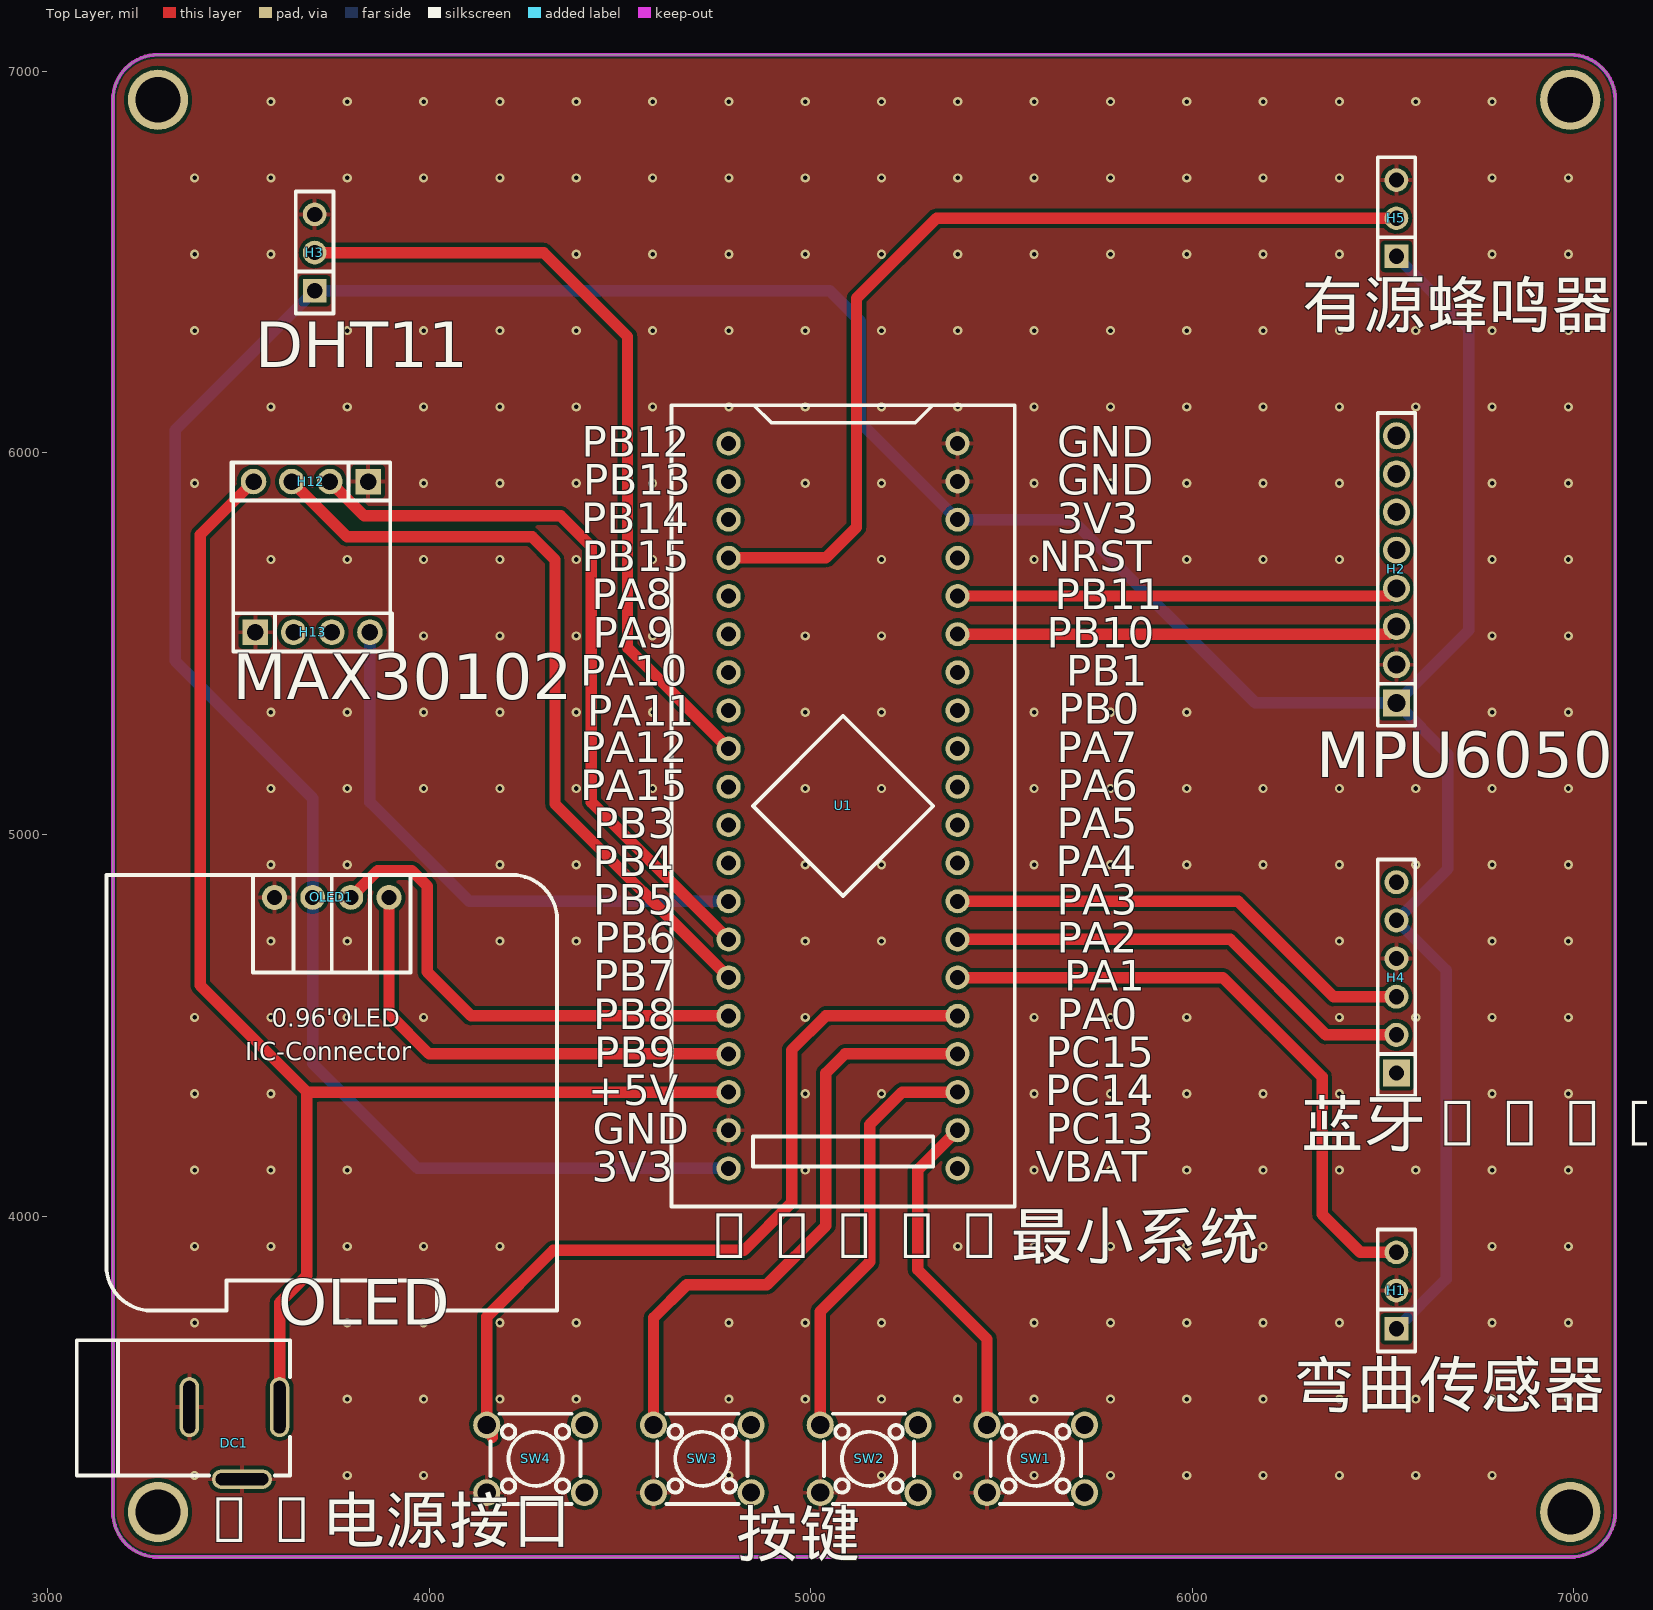
[diagram p0: Top Layer view]
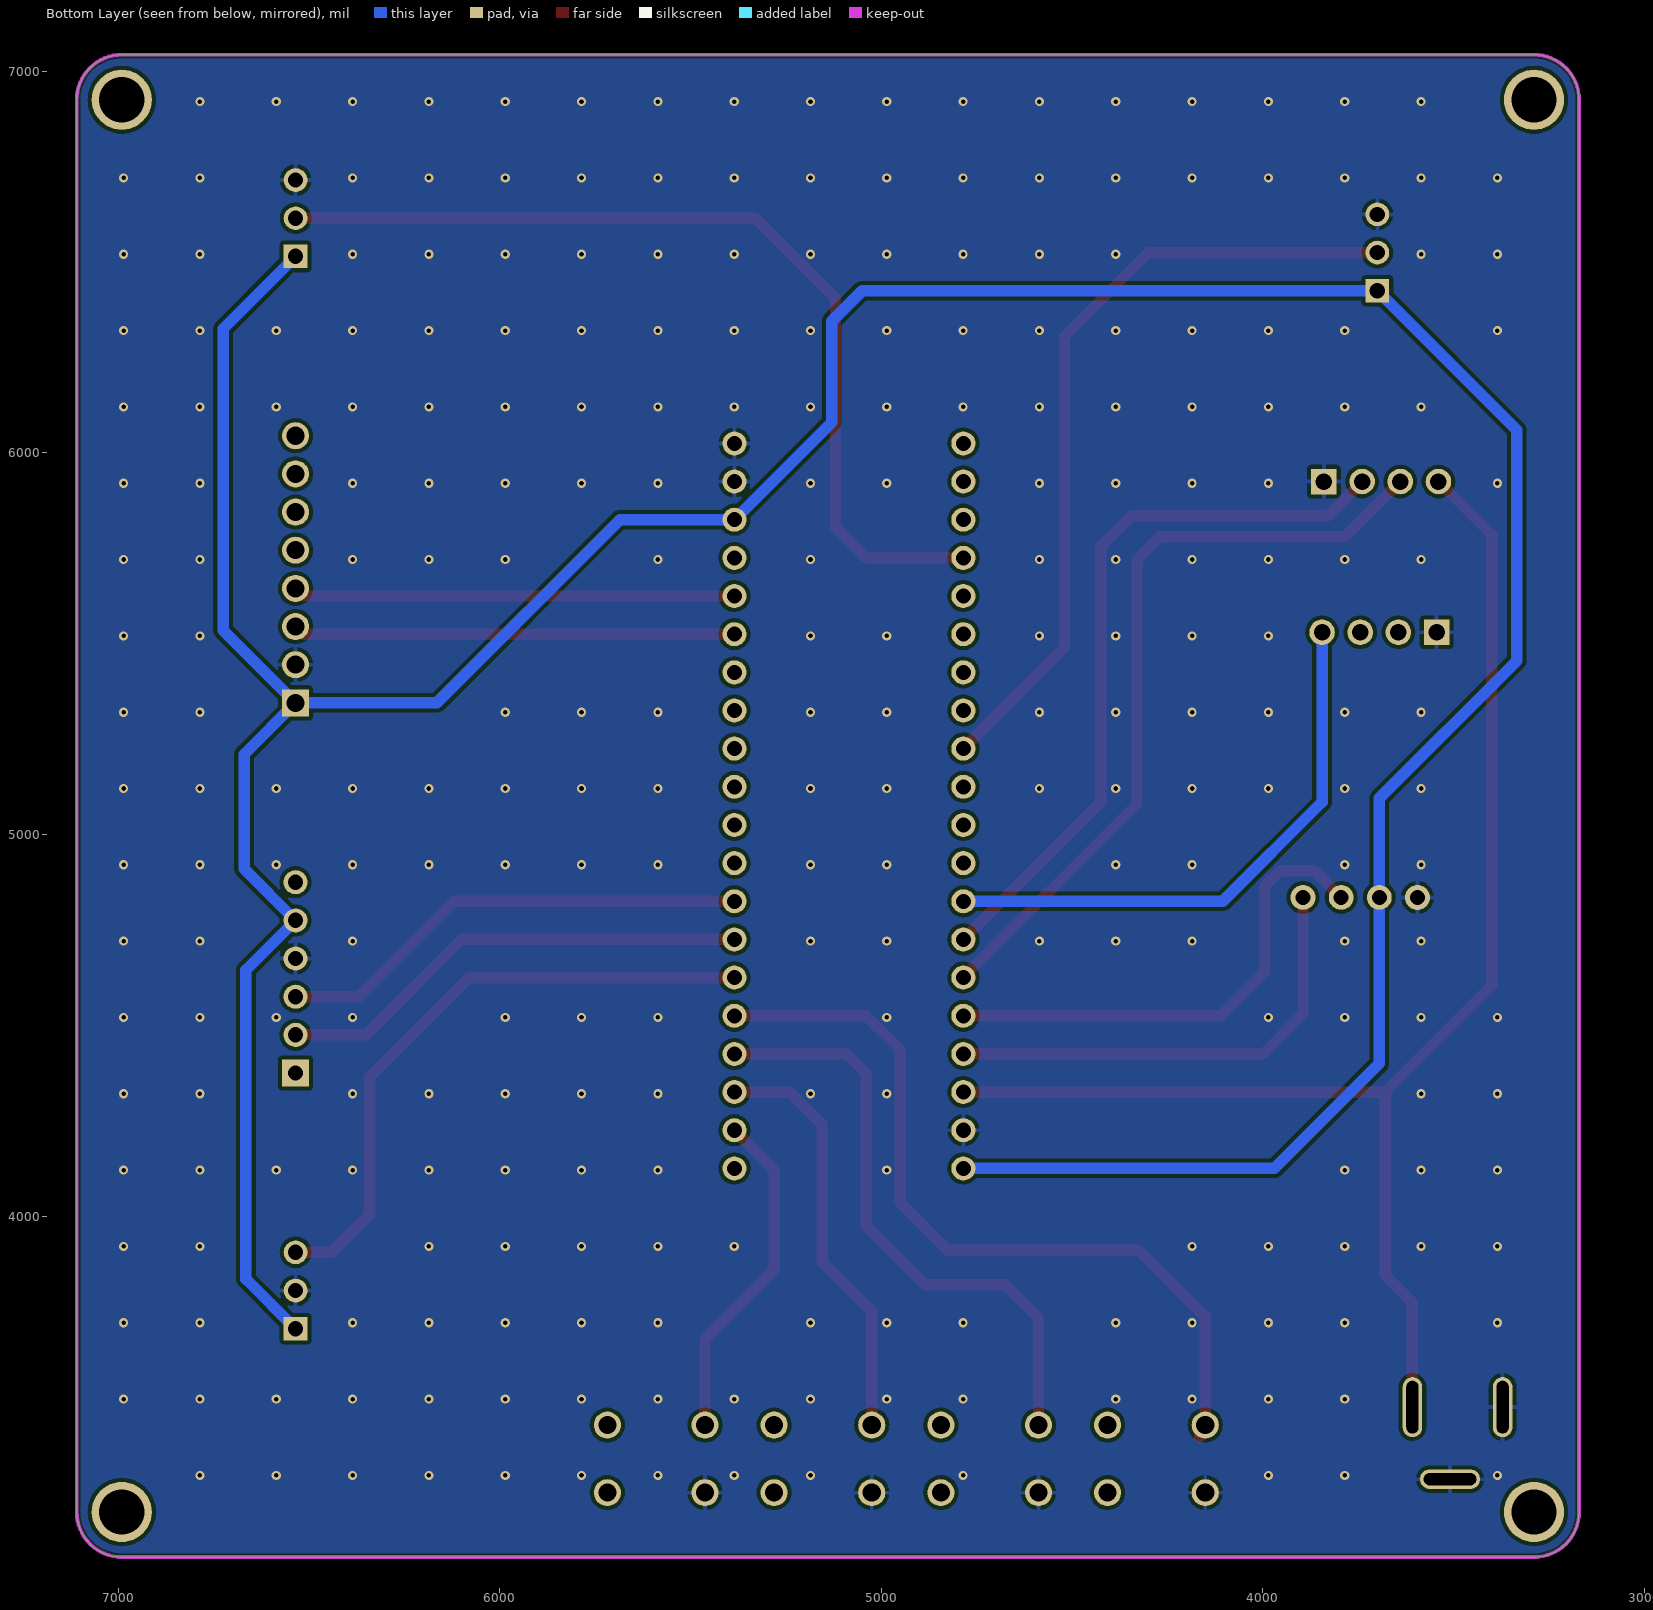
[diagram p1: Bottom Layer view, seen from below]
# Altium PCB MISC51890.pcbdoc
Units mil, origin at the board's own origin, x right, y up, seen from the top; angles counter-clockwise.
Board outline 3937.01 x 3937.01 mil, 2 copper layers (Top Layer, Bottom Layer), stack 62.206 mil thick; 14 components, 37 nets, 98 pads, 265 vias.

## Layer stack, top to bottom
Top Solder Mask Layer: solder mask 0.394, Dk 3.3
Top Layer: signal copper 1.379
Dielectric1: surface 59.449, FR4, Dk 4.5
Bottom Layer: signal copper 1.378
Bottom Solder Mask Layer: solder mask 0.394, Dk 3.3

## Board outline
6990.39,3106.5 ccw(c6990.39,3224.61) 7108.5,3224.61 7108.5,6925.39 ccw(c6990.39,6925.39) 6990.39,7043.5 3289.61,7043.5 ccw(c3289.61,6925.39) 3171.5,6925.39 3171.5,3224.61 ccw(c3289.61,3224.61) 3289.61,3106.5

## Design rules (kind name [scope] priority, off if disabled: settings)
BoardOutlineClearance copperThickness2oz_1 [All] p2 off: genericclearance=7.99 ignorepadtopadclearanceinfootprint=FALSE except(0: Arc-SplitContinuation Track-SplitContinuation SMDPad-SplitContinuation THPad-SplitContinuation Via-SplitContinuation Fill-SplitContinuation Region-SplitContinuation Poly-SplitContinuation Text-SplitContinuation Hole-SplitContinuation; 5.98: Arc-CutoutEdge Track-CutoutEdge SMDPad-CutoutEdge THPad-CutoutEdge Via-CutoutEdge Text-CutoutEdge; 6.89: Hole-OutlineEdge Hole-CutoutEdge; 10: Poly-OutlineEdge Poly-CutoutEdge; 11.81: Arc-OutlineEdge Track-OutlineEdge SMDPad-OutlineEdge THPad-OutlineEdge Via-OutlineEdge Fill-OutlineEdge Region-OutlineEdge Text-OutlineEdge Fill-CutoutEdge Region-CutoutEdge)
BoardOutlineClearance Plane_innerPlane_1 [All] p4 off: genericclearance=4.02 ignorepadtopadclearanceinfootprint=FALSE except(0: Arc-SplitContinuation Track-SplitContinuation SMDPad-SplitContinuation THPad-SplitContinuation Via-SplitContinuation Fill-SplitContinuation Region-SplitContinuation Poly-SplitContinuation Text-SplitContinuation Hole-SplitContinuation; 5.98: Arc-CutoutEdge Track-CutoutEdge SMDPad-CutoutEdge THPad-CutoutEdge Via-CutoutEdge Text-CutoutEdge; 6.89: Hole-OutlineEdge Hole-CutoutEdge; 10: Poly-OutlineEdge Poly-CutoutEdge; 11.81: Arc-OutlineEdge Track-OutlineEdge SMDPad-OutlineEdge THPad-OutlineEdge Via-OutlineEdge Fill-OutlineEdge Region-OutlineEdge Text-OutlineEdge Fill-CutoutEdge Region-CutoutEdge)
BoardOutlineClearance Copper_copperRegion_1 [All] p6 off: genericclearance=4.02 ignorepadtopadclearanceinfootprint=FALSE except(0: Arc-SplitContinuation Track-SplitContinuation SMDPad-SplitContinuation THPad-SplitContinuation Via-SplitContinuation Fill-SplitContinuation Region-SplitContinuation Poly-SplitContinuation Text-SplitContinuation Hole-SplitContinuation; 5.98: Arc-CutoutEdge Track-CutoutEdge SMDPad-CutoutEdge THPad-CutoutEdge Via-CutoutEdge Text-CutoutEdge; 6.89: Hole-OutlineEdge Hole-CutoutEdge; 10: Poly-OutlineEdge Poly-CutoutEdge; 11.81: Arc-OutlineEdge Track-OutlineEdge SMDPad-OutlineEdge THPad-OutlineEdge Via-OutlineEdge Fill-OutlineEdge Region-OutlineEdge Text-OutlineEdge Fill-CutoutEdge Region-CutoutEdge)
BoardOutlineClearance copperThickness1oz_1 [All] p8: genericclearance=4.02 ignorepadtopadclearanceinfootprint=FALSE except(0: Arc-SplitContinuation Track-SplitContinuation SMDPad-SplitContinuation THPad-SplitContinuation Via-SplitContinuation Fill-SplitContinuation Region-SplitContinuation Poly-SplitContinuation Text-SplitContinuation Hole-SplitContinuation; 5.98: Arc-CutoutEdge Track-CutoutEdge SMDPad-CutoutEdge THPad-CutoutEdge Via-CutoutEdge Text-CutoutEdge; 6.89: Hole-OutlineEdge Hole-CutoutEdge; 10: Poly-OutlineEdge Poly-CutoutEdge; 11.81: Arc-OutlineEdge Track-OutlineEdge SMDPad-OutlineEdge THPad-OutlineEdge Via-OutlineEdge Fill-OutlineEdge Region-OutlineEdge Text-OutlineEdge Fill-CutoutEdge Region-CutoutEdge)
Clearance copperThickness2oz [All] p1 off: gap=7.99 ignorepadtopadclearanceinfootprint=FALSE except(5.98: SMDPad-Track SMDPad-SMDPad THPad-Track SMDPad-THPad THPad-THPad Track-Via SMDPad-Via THPad-Via Via-Via Fill-SMDPad Region-SMDPad Fill-THPad Region-THPad Fill-Via Region-Via Fill-Fill Fill-Region Region-Region Arc-Track Arc-SMDPad Arc-THPad Arc-Via Fill-Arc Region-Arc Arc-Arc Text-Track SMDPad-Text Text-THPad Text-Via Fill-Text Region-Text Arc-Text Text-Text; 6.89: Hole-Track Hole-SMDPad Hole-THPad Hole-Via Fill-Hole Region-Hole Hole-Arc Hole-Text; 10: Poly-Track Poly-SMDPad Poly-THPad Poly-Via Poly-Fill Poly-Region Poly-Poly Poly-Arc Poly-Text Poly-Hole; 11.81: Fill-Track Region-Track)
Clearance Plane_innerPlane [All] p3 off: gap=4.02 ignorepadtopadclearanceinfootprint=FALSE except(5.98: SMDPad-Track SMDPad-SMDPad THPad-Track SMDPad-THPad THPad-THPad Track-Via SMDPad-Via THPad-Via Via-Via Fill-SMDPad Region-SMDPad Fill-THPad Region-THPad Fill-Via Region-Via Fill-Fill Fill-Region Region-Region Arc-Track Arc-SMDPad Arc-THPad Arc-Via Fill-Arc Region-Arc Arc-Arc Text-Track SMDPad-Text Text-THPad Text-Via Fill-Text Region-Text Arc-Text Text-Text; 6.89: Hole-Track Hole-SMDPad Hole-THPad Hole-Via Fill-Hole Region-Hole Hole-Arc Hole-Text; 10: Poly-Track Poly-SMDPad Poly-THPad Poly-Via Poly-Fill Poly-Region Poly-Poly Poly-Arc Poly-Text Poly-Hole; 11.81: Fill-Track Region-Track)
Clearance Copper_copperRegion [All] p5 off: gap=4.02 ignorepadtopadclearanceinfootprint=FALSE except(5.98: SMDPad-Track SMDPad-SMDPad THPad-Track SMDPad-THPad THPad-THPad Track-Via SMDPad-Via THPad-Via Via-Via Fill-SMDPad Region-SMDPad Fill-THPad Region-THPad Fill-Via Region-Via Fill-Fill Fill-Region Region-Region Arc-Track Arc-SMDPad Arc-THPad Arc-Via Fill-Arc Region-Arc Arc-Arc Text-Track SMDPad-Text Text-THPad Text-Via Fill-Text Region-Text Arc-Text Text-Text; 6.89: Hole-Track Hole-SMDPad Hole-THPad Hole-Via Fill-Hole Region-Hole Hole-Arc Hole-Text; 10: Poly-Track Poly-SMDPad Poly-THPad Poly-Via Poly-Fill Poly-Region Poly-Poly Poly-Arc Poly-Text Poly-Hole; 11.81: Fill-Track Region-Track)
Clearance copperThickness1oz [All] p7: gap=4.02 ignorepadtopadclearanceinfootprint=FALSE except(5.98: SMDPad-Track SMDPad-SMDPad THPad-Track SMDPad-THPad THPad-THPad Track-Via SMDPad-Via THPad-Via Via-Via Fill-SMDPad Region-SMDPad Fill-THPad Region-THPad Fill-Via Region-Via Fill-Fill Fill-Region Region-Region Arc-Track Arc-SMDPad Arc-THPad Arc-Via Fill-Arc Region-Arc Arc-Arc Text-Track SMDPad-Text Text-THPad Text-Via Fill-Text Region-Text Arc-Text Text-Text; 6.89: Hole-Track Hole-SMDPad Hole-THPad Hole-Via Fill-Hole Region-Hole Hole-Arc Hole-Text; 10: Poly-Track Poly-SMDPad Poly-THPad Poly-Via Poly-Fill Poly-Region Poly-Poly Poly-Arc Poly-Text Poly-Hole; 11.81: Fill-Track Region-Track)
DiffPairsRouting differentialPair [All] p1: maxlimit=6 minlimit=6 mostfreqgap=6 toplayer_minwidth=5 toplayer_prefwidth=10 toplayer_maxwidth=100 toplayer_mingap=6 toplayer_prefgap=6 toplayer_maxgap=6 bottomlayer_minwidth=5 bottomlayer_prefwidth=10 bottomlayer_maxwidth=100 bottomlayer_mingap=6 bottomlayer_prefgap=6 bottomlayer_maxgap=6 maxuncoupledlength=10
HoleToHoleClearance otherClearance [All] p1: gap=11.81 allowstackedmicrovias=TRUE
Length netLength [All] p1: minlimit=0 maxlimit=0
PasteMaskExpansion pasteMaskExpansion [All] p1: expansion=0
PlaneConnect innerPlane [All] p1: planeconnectstyle=Relief reliefexpansion=20 reliefentries=4 reliefconductorwidth=10 reliefairgap=10
PolygonConnect copperRegion [All] p1: connectstyle=Relief reliefconductorwidth=10 reliefentries=4 polygonreliefangle="90 Angle" airgapwidth=10 via.connectstyle=Relief via.reliefconductorwidth=10 via.reliefentries=4 via.polygonreliefangle="90 Angle" via.airgapwidth=10
RoutingVias viaSize [All] p1: holewidth=12.01 width=24.02 viastyle="Through Hole" minholewidth=11.81 minwidth=19.68 maxholewidth=248.03 maxwidth=393.7
SolderMaskExpansion solderMaskExpansion [IsVia] p1: expansion=-1000 istentingtop=TRUE
SolderMaskExpansion solderMaskExpansion [All] p2: expansion=2.01 istentingtop=FALSE
Width copperThickness2oz_2 [All] p1 off: maxlimit=100 minlimit=8 preferedwidth=10
Width copperThickness1oz_2 [All] p2: maxlimit=100 minlimit=5 preferedwidth=30

## Components (designator, comment, footprint, x,y, rotation, side; value= is the part's Value field where it differs from the comment)
DC1 "" DC-2.0 3485,3510 r180 top
H1 "" HDR-TH_3P-P2.54-V-F 6535,3805 r90 top
H2 "" HDR-TH_8P-P2.54-V-F-1 6535,5695 r90 top
H3 "" HDR-TH_3P-P2.54-V-F 3700,6525 r90 top
H4 "" HDR-TH_6P-P2.54-V-F 6535,4625 r90 top
H5 "" HDR-TH_3P-P2.54-V-F 6535,6615 r90 top
H12 "" HDR-TH_4P-P2.54-V-F 3690,5925 r180 top
H13 "" HDR-TH_4P-P2.54-V-F 3695,5530 r0 top
OLED1 "" 0.96OLED_4P 3745,4835 r0 top
SW1 "" SW-TH_4P-L6.0-W6.0-P4.50-LS6.5 5590,3363.89 r0 top
SW2 "" SW-TH_4P-L6.0-W6.0-P4.50-LS6.5 5153.02,3363.89 r0 top
SW3 "" SW-TH_4P-L6.0-W6.0-P4.50-LS6.5 4716.04,3363.89 r0 top
SW4 "" SW-TH_4P-L6.0-W6.0-P4.50-LS6.5 4279.06,3363.89 r0 top
U1 "STM32F103C8T6-Card" CONN-TH_L53.3-W22.9_STM32F103C8T6-CARD 5085,5075 r270 top

## Footprints (in the part's own frame and the unit in brackets; to place one, negate y for a bottom-side part, rotate by r counter-clockwise, add the part's x,y. Pads: shape width x height; smd on the part's side, far side on the other; paste and mask are expansions set on the pad)
0.96OLED_4P [mm]
  round 1.65 hole 1 copper offset 0,0: 1(-3.81,-0.001) 2(-1.27,0.002) 3(1.27,0.002) 4(3.81,0.002)
  silkscreen extent -15,-27.5 15,1.5
CONN-TH_L53.3-W22.9_STM32F103C8T6-CARD [mm]
  round 1.6 hole 1: 1(-24.13,-7.62) 2(-21.59,-7.62) 3(-19.05,-7.62) 4(-16.51,-7.62) 5(-13.97,-7.62) 6(-11.43,-7.62) 7(-8.89,-7.62) 8(-6.35,-7.62) 9(-3.81,-7.62) 10(-1.27,-7.62) 11(1.27,-7.62) 12(3.81,-7.62) 13(6.35,-7.62) 14(8.89,-7.62) 15(11.43,-7.62) 16(13.97,-7.62) 17(16.51,-7.62) 18(19.05,-7.62) 19(21.59,-7.62) 20(24.13,-7.62) 21(24.13,7.62) 22(21.59,7.62) 23(19.05,7.62) 24(16.51,7.62) 25(13.97,7.62) 26(11.43,7.62) 27(8.89,7.62) 28(6.35,7.62) 29(3.81,7.62) 30(1.27,7.62) 31(-1.27,7.62) 32(-3.81,7.62) 33(-6.35,7.62) 34(-8.89,7.62) 35(-11.43,7.62) 36(-13.97,7.62) 37(-16.51,7.62) 38(-19.05,7.62) 39(-21.59,7.62) 40(-24.13,7.62)
  silkscreen extent -26.67,-11.43 26.67,11.43
DC-2.0 [mil]
  oval 157.5x51.2 hole 31.5 slot 137.8 at 0 deg paste+0 mask+2: 2(-24.7,199.5)
  oval 51.2x157.5 hole 31.5 slot 137.8 at 90 deg paste+0 mask+2: 3(113.1,10.5) 4(-123.1,10.5)
  silkscreen extent -151,-165 408,190
HDR-TH_3P-P2.54-V-F [mil]
  rect 62x62 hole 40.16: 1(-100,0)
  round 62 hole 40.16: 2(0,0) 3(100,0)
  silkscreen extent -160,-49 160,49
HDR-TH_4P-P2.54-V-F [mm]
  rect 1.7x1.7 hole 1.1: 1(-3.81,0)
  round 1.7 hole 1.1: 2(-1.27,0) 3(1.27,0) 4(3.81,0)
  silkscreen extent -5.29,-1.27 5.29,1.27
HDR-TH_6P-P2.54-V-F [mm]
  rect 1.8x1.8 hole 1.02: 1(-6.35,0)
  round 1.6 hole 1.02: 2(-3.81,0) 3(-1.27,0) 4(1.27,0) 5(3.81,0) 6(6.35,0)
  silkscreen extent -7.87,-1.25 7.87,1.25
HDR-TH_8P-P2.54-V-F-1 [mm]
  rect 1.8x1.8 hole 1.2: 1(-8.89,0)
  round 1.8 hole 1.2: 2(-6.35,0) 3(-3.81,0) 4(-1.27,0) 5(1.27,0) 6(3.81,0) 7(6.35,0) 8(8.89,0)
  silkscreen extent -10.41,-1.25 10.41,1.25
SW-TH_4P-L6.0-W6.0-P4.50-LS6.5 [mm]
  round 1.8 hole 1.2: 1(-3.25,2.25) 2(3.25,2.25) 3(-3.25,-2.25) 4(3.25,-2.25)
  silkscreen extent -3,-3 3,3

## Free pads (board coordinates)
  round 157.48 hole 118.11: 1(3289.61,6925.39) 1(3289.61,3224.61) 1(6990.39,6925.39) 1(6990.39,3224.61)

## Via types
v1: diameter 24.02, hole 12, Top Layer to Bottom Layer, 265 vias

## Nets (pads, with @x,y where several pads share a name; then routed paths per layer and width w, separated by ;. In a path a pad name is that pad's centre, name@x,y a point inside that pad or via, vN(x,y) a via of type N, cw(c..) or ccw(c..) an arc to the next point about the centre after c; other vN are vias at no path point)
+5V: DC1.4 H12.4 U1.18 | length 3734.3
  Top Layer w30: H12.4 3400,5785 3400,4605 3680,4325 ; DC1.4 3608.1,3773.1 3680,3845 3680,4325 ; U1.18 3680,4325
GND: DC1.2 DC1.3 H1.2 H2.2 H3.3 H4.4 H5.3 H12.1 H13.1 OLED1.1 SW1.3 SW2.3 SW3.3 SW4.3 U1.19 U1.39 U1.40
  other v1: 3385.6,3320.6 3785.6,3320.6 3985.6,3320.6 4785.6,3320.6 5185.6,3320.6 5385.6,3320.6 5585.6,3320.6 5785.6,3320.6 5985.6,3320.6 6185.6,3320.6 6385.6,3320.6 6585.6,3320.6 6785.6,3320.6 3785.6,3520.6 3985.6,3520.6 4185.6,3520.6 4385.6,3520.6 4785.6,3520.6 4985.6,3520.6 5185.6,3520.6 5385.6,3520.6 5585.6,3520.6 5785.6,3520.6 5985.6,3520.6 6185.6,3520.6 6385.6,3520.6 6585.6,3520.6 6785.6,3520.6 6985.6,3520.6 3385.6,3720.6 3785.6,3720.6 3985.6,3720.6 4185.6,3720.6 4385.6,3720.6 4785.6,3720.6 4985.6,3720.6 5185.6,3720.6 5585.6,3720.6 5785.6,3720.6 5985.6,3720.6 6185.6,3720.6 6385.6,3720.6 6785.6,3720.6 6985.6,3720.6 3385.6,3920.6 3585.6,3920.6 3785.6,3920.6 3985.6,3920.6 4185.6,3920.6 5385.6,3920.6 5585.6,3920.6 5785.6,3920.6 5985.6,3920.6 6185.6,3920.6 6785.6,3920.6 6985.6,3920.6 3385.6,4120.6 3585.6,4120.6 3785.6,4120.6 4985.6,4120.6 5585.6,4120.6 5785.6,4120.6 5985.6,4120.6 6185.6,4120.6 6385.6,4120.6 6585.6,4120.6 6785.6,4120.6 6985.6,4120.6 3385.6,4320.6 3585.6,4320.6 4985.6,4320.6 5185.6,4320.6 5585.6,4320.6 5785.6,4320.6 5985.6,4320.6 6185.6,4320.6 6385.6,4320.6 6785.6,4320.6 6985.6,4320.6 3385.6,4520.6 3585.6,4520.6 3785.6,4520.6 3985.6,4520.6 4985.6,4520.6 5585.6,4520.6 5785.6,4520.6 5985.6,4520.6 6385.6,4520.6 6585.6,4520.6 6785.6,4520.6 6985.6,4520.6 3585.6,4720.6 3785.6,4720.6 4185.6,4720.6 4385.6,4720.6 4585.6,4720.6 4985.6,4720.6 5185.6,4720.6 6385.6,4720.6 6785.6,4720.6 6985.6,4720.6 3585.6,4920.6 3785.6,4920.6 4185.6,4920.6 4385.6,4920.6 4985.6,4920.6 5185.6,4920.6 5585.6,4920.6 5785.6,4920.6 5985.6,4920.6 6185.6,4920.6 6385.6,4920.6 6585.6,4920.6 6785.6,4920.6 6985.6,4920.6 3585.6,5120.6 3785.6,5120.6 3985.6,5120.6 4185.6,5120.6 4385.6,5120.6 4585.6,5120.6 4985.6,5120.6 5185.6,5120.6 5585.6,5120.6 5785.6,5120.6 5985.6,5120.6 6185.6,5120.6 6385.6,5120.6 6585.6,5120.6 6785.6,5120.6 6985.6,5120.6 3585.6,5320.6 3785.6,5320.6 3985.6,5320.6 4185.6,5320.6 4385.6,5320.6 4585.6,5320.6 4985.6,5320.6 5185.6,5320.6 5585.6,5320.6 5785.6,5320.6 5985.6,5320.6 6785.6,5320.6 6985.6,5320.6 3985.6,5520.6 4185.6,5520.6 4385.6,5520.6 4585.6,5520.6 4985.6,5520.6 5185.6,5520.6 6785.6,5520.6 6985.6,5520.6 3585.6,5720.6 3785.6,5720.6 3985.6,5720.6 4185.6,5720.6 4385.6,5720.6 4585.6,5720.6 5185.6,5720.6 5585.6,5720.6 5985.6,5720.6 6185.6,5720.6 6385.6,5720.6 6785.6,5720.6 6985.6,5720.6 3385.6,5920.6 3985.6,5920.6 4185.6,5920.6 4385.6,5920.6 4585.6,5920.6 4985.6,5920.6 5185.6,5920.6 5585.6,5920.6 5785.6,5920.6 5985.6,5920.6 6185.6,5920.6 6385.6,5920.6 6785.6,5920.6 6985.6,5920.6 3585.6,6120.6 3785.6,6120.6 3985.6,6120.6 4185.6,6120.6 4385.6,6120.6 4585.6,6120.6 4785.6,6120.6 4985.6,6120.6 5185.6,6120.6 5385.6,6120.6 5585.6,6120.6 5785.6,6120.6 5985.6,6120.6 6185.6,6120.6 6385.6,6120.6 6585.6,6120.6 6785.6,6120.6 6985.6,6120.6 3385.6,6320.6 3785.6,6320.6 3985.6,6320.6 4185.6,6320.6 4385.6,6320.6 4585.6,6320.6 4785.6,6320.6 4985.6,6320.6 5185.6,6320.6 5385.6,6320.6 5585.6,6320.6 5785.6,6320.6 5985.6,6320.6 6185.6,6320.6 6385.6,6320.6 6585.6,6320.6 6785.6,6320.6 6985.6,6320.6 3385.6,6520.6 3585.6,6520.6 4385.6,6520.6 4585.6,6520.6 4785.6,6520.6 4985.6,6520.6 5185.6,6520.6 5385.6,6520.6 5585.6,6520.6 5785.6,6520.6 5985.6,6520.6 6185.6,6520.6 6385.6,6520.6 6785.6,6520.6 6985.6,6520.6 3385.6,6720.6 3585.6,6720.6 3785.6,6720.6 3985.6,6720.6 4185.6,6720.6 4385.6,6720.6 4585.6,6720.6 4785.6,6720.6 4985.6,6720.6 5185.6,6720.6 5385.6,6720.6 5585.6,6720.6 5785.6,6720.6 5985.6,6720.6 6185.6,6720.6 6385.6,6720.6 6785.6,6720.6 6985.6,6720.6 3585.6,6920.6 3785.6,6920.6 3985.6,6920.6 4185.6,6920.6 4385.6,6920.6 4585.6,6920.6 4785.6,6920.6 4985.6,6920.6 5185.6,6920.6 5385.6,6920.6 5585.6,6920.6 5785.6,6920.6 5985.6,6920.6 6185.6,6920.6 6385.6,6920.6 6585.6,6920.6 6785.6,6920.6
NRST: U1.37
PA0: SW4.1 U1.25 | length 2111.1
  Top Layer w30: SW4.1 4151.11,3736.11 4325,3910 4825,3910 4950,4035 4950,4435 5040,4525 U1.25 ; SW4.1@4165,3420 SW4.1@4165,3452.47
PA1: H1.3 U1.26 | length 1659.1
  Top Layer w30: U1.26 6080,4625 6340,4365 6340,4005 6440,3905 H1.3
PA2: H4.2 U1.27 | length 1253.6
  Top Layer w30: U1.27 6100,4725 6350,4475 H4.2
PA3: H4.3 U1.28 | length 1253.6
  Top Layer w30: U1.28 6120,4825 6370,4575 H4.3
PA4: U1.29
PA5: U1.30
PA6: U1.31
PA7: U1.32
PA8: U1.5
PA9: U1.6
PA10: U1.7
PA11: U1.8
PA12: H3.2 U1.9 | length 2100.9
  Top Layer w30: H3.2 4300,6525 4520,6305 4520,5490 U1.9
PA15: U1.10
PB0: U1.33
PB1: U1.34
PB3: U1.11
PB4: U1.12
PB5: H13.4 U1.13 | length 1492.7
  Bottom Layer w30: H13.4 3845,5085 4105,4825 U1.13
PB6: H12.2 U1.14 | length 1934.5
  Top Layer w30: H12.2 3830,5835 4345,5835 4425,5755 4425,5085 U1.14
PB7: H12.3 U1.15 | length 2058.4
  Top Layer w30: H12.3 3785,5780 4270,5780 4330,5720 4330,5080 U1.15
PB8: OLED1.3 U1.16 | length 1308.2
  Top Layer w30: OLED1.3@3795,4835.05 3864.95,4905 3955,4905 3995,4865 3995,4640 4110,4525 U1.16
PB9: OLED1.4 U1.17 | length 1238.5
  Top Layer w30: OLED1.4@3895,4835.05 3895,4530 4000,4425 U1.17
PB10: H2.3 U1.35 | length 1158.3
  Top Layer w30: U1.35 6515,5525 H2.3
PB11: H2.4 U1.36 | length 1158.3
  Top Layer w30: U1.36 6515,5625 H2.4
PB12: U1.1
PB13: U1.2
PB14: U1.3
PB15: H5.2 U1.4 | length 2470.1
  Top Layer w30: U1.4 5040,5725 5120,5805 5120,6405 5330,6615 H5.2
PC13: SW1.1 U1.22 | length 891.4
  Top Layer w30: U1.22 5280,4120 5280,3860 5462.05,3677.95 SW1.1
PC14: SW2.1 U1.23 | length 1106.6
  Top Layer w30: SW2.1 5025.07,3750.07 5155,3880 5155,4240 5240,4325 U1.23
PC15: SW3.1 U1.24 | length 1598.4
  Top Layer w30: SW3.1 4588.09,3733.09 4675,3820 4885,3820 5040,3975 5040,4375 5090,4425 U1.24
VBAT: U1.21
VCC: H1.1 H2.1 H3.1 H4.5 H5.1 OLED1.2 U1.20 U1.38 | length 10153.7
  Bottom Layer w30: U1.20 3970,4125 3695,4400 3695,4835.05 3695,5095 3335,5455 3335,6060 H3.1 5050,6425 5130,6345 5130,6080 U1.38 5685,5825 6165,5345 H2.1 ; H1.1 6665,3835 6665,4645 H4.5 6670,4910 6670,5210 H2.1 ; H5.1 6725,6325 6725,5535 H2.1
pads on no net: H2.5 H2.6 H2.7 H2.8 H4.1 H4.6 H13.2 H13.3 SW1.2 SW1.4 SW2.2 SW2.4 SW3.2 SW3.4 SW4.2 SW4.4

## Polygon pours and split planes (outlines as drawn)
GND on Bottom Layer (solid, remove dead copper, pour order 2): 3100,7165 3100,3000 7275,3000 7275,7165
GND on Top Layer (solid, remove dead copper, pour order 0): 3000,7145 3000,3075 7385,3075 7385,7145

## Keep-outs
Board Outline Layer:
  the board outline again, w10

## Silkscreen, mask and mechanical layers (free items; w line width, h text height)
Top Silkscreen Layer:
  lines w10: 3486.73,5480 3898.27,5480 3898.27,5975 3486.73,5975 3486.73,5480
  text "有源蜂鸣器" at 6285,6330 h120
  text "DHT11" at 3545,6225 h120
  text "PB12" at 4400.64,5990 h80
  text "GND" at 5646.65,5990 h80
  text "PB13" at 4403.85,5890 h80
  text "GND" at 5646.65,5890 h80
  text "PB14" at 4398.34,5790 h80
  text "3V3" at 5644.45,5790 h80
  text "PB15" at 4400.64,5690 h80
  text "NRST" at 5598.65,5690 h80
  text "PA8" at 4426.24,5590 h80
  text "PB11" at 5639.05,5590 h80
  text "PA9" at 4428.44,5490 h80
  text "PB10" at 5618.85,5490 h80
  text "PA10" at 4396.14,5390 h80
  text "PB1" at 5669.15,5390 h80
  text "MAX30102" at 3485,5355 h120
  text "PB0" at 5648.95,5290 h80
  text "PA11" at 4414.55,5285 h80
  text "PA12" at 4396.14,5190 h80
  text "PA7" at 5644.45,5190 h80
  text "MPU6050" at 6325,5150 h120
  text "PA15" at 4396.14,5090 h80
  text "PA6" at 5646.65,5090 h80
  text "PB3" at 4430.74,4990 h80
  text "PA5" at 5644.45,4990 h80
  text "PB4" at 4428.44,4890 h80
  text "PA4" at 5642.15,4890 h80
  text "PB5" at 4430.74,4790 h80
  text "PA3" at 5644.45,4790 h80
  text "PB6" at 4432.94,4690 h80
  text "PA2" at 5644.45,4690 h80
  text "PB7" at 4430.74,4590 h80
  text "PA1" at 5664.65,4590 h80
  text "PB8" at 4430.74,4490 h80
  text "PA0" at 5644.45,4490 h80
  text "PB9" at 4432.94,4390 h80
  text "PC15" at 5616.55,4390 h80
  text "+5V" at 4417.24,4290 h80
  text "PC14" at 5614.25,4290 h80
  text "GND" at 4428.44,4190 h80
  text "PC13" at 5616.55,4190 h80
  text "蓝牙HC-05" at 6285,4185 h120
  text "3V3" at 4426.24,4090 h80
  text "VBAT" at 5589.65,4090 h80
  text "STM32最小系统" at 4705,3890 h120
  text "OLED" at 3605,3715 h120
  text "弯曲传感器" at 6265,3500 h120
  text "DC电源接口" at 3395,3145 h120
  text "按键" at 4805,3110 h120